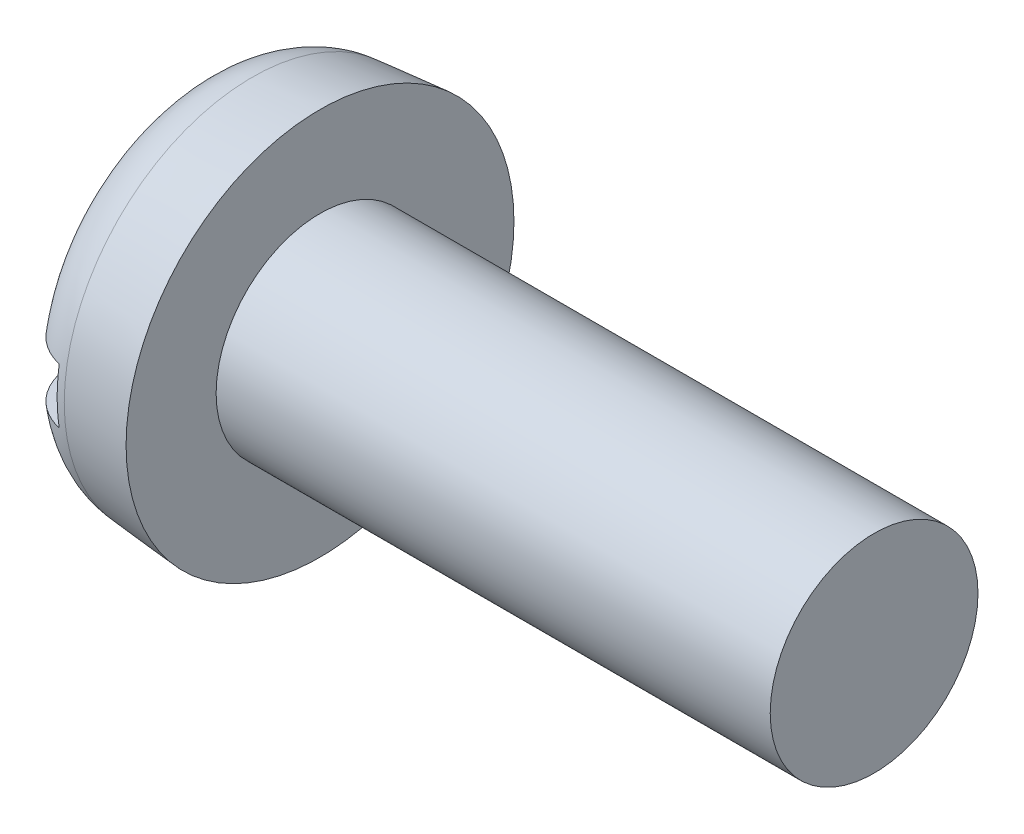
SolidWorks part; units mm, degrees
ref_plane "Plane1" through (0, 0, 0) normal (0, 0, 1) x (1, 0, 0)
ref_plane "Plane2" through (0, 0, 0) normal (0, 1, 0) x (1, 0, 0)
ref_plane "Plane3" through (0, 0, 0) normal (1, 0, 0) x (0, 0, -1)
sketch "BodySke" plane through (0, 0, 0) normal (0, 0, 1) x (1, 0, 0)
  line L0 (1.8, 1.5) -> (1.8, 2.8)
  line L1 (0, 0) -> (0, 2.6425)
  line L2 (-25.4, 0) -> (127, 0) construction
  line L3 (9.8, 0) -> (0, 0)
  line L4 (1.8, 1.5) -> (9.8, 1.5)
  line L5 (9.8, 1.5) -> (9.8, 0)
  line L6 (0, 2.6425) -> (1.8, 2.8)
  line L9 (2.3, 3.0875) -> (2.3, -6.4375) construction
  line L10 (1.8, 6.35) -> (1.8, -3.175) construction
revolve "Base-Revolve" add sketch "BodySke"
cosmetic thread "ThreadCosmetic" [suppressed]
fillet "Fillet1" [suppressed] radius 0.1
fillet "Fillet2" radius 0.9 1 edges at (0, 0, 2.6425)
sketch "Sketch2" plane through (0, 0, 0) normal (1, 0, 0) x (0, 0, -1)
  line L0 (2.8, -0.4) -> (-2.8, -0.4)
  line L1 (2.8, -0.4) -> (2.8, 0.4)
  line L2 (-2.8, 0.4) -> (2.8, 0.4)
  line L3 (-2.8, 0.4) -> (-2.8, -0.4)
extrude "Slot" cut sketch "Sketch2" along normal blind 0.7
sketch "ThdSchSke" plane through (0, 0, 0) normal (0, 0, 1) x (1, 0, 0)
  line L0 (2.8, -1.2195) -> (2.6036, -1.5)
  line L1 (2.8, -1.2195) -> (2.9964, -1.5)
  line L2 (2.9964, -1.5) -> (2.9964, -1.875)
  line L3 (-3.175, 0) -> (5.1513, 0) construction
  line L5 (2.9964, -1.875) -> (2.6036, -1.875)
  line L6 (2.6036, -1.875) -> (2.6036, -1.5)
revolve "ThreadSchematic" [suppressed] cut sketch "ThdSchSke" angle 360 about L3
pattern_linear "ThdSchPat" [suppressed]
equation "\"D1@Sketch2\" = \"Head_dia@BodySke\""
equation "\"D2@Sketch2\" = \"D1@Sketch2\" / 2"
equation "\"D3@Sketch2\" = \"Slot_width@Sketch2\" / 2"
equation "\"Thread_length@ThreadCosmetic\" = ((sgn( (\"Length@BodySke\" - \"Advance@BodySke\" * 2.0 ) - \"Thread_nom@BodySke\" )-1)*( (\"Length@BodySke\" - \"Advance@BodySke\"  * 2.0) - \"Thread_nom@BodySke\" ))/-2+ \"Thread_nom@BodySke\""
equation "\"Thread_minor@ThdSchSke\" = \"Thread_minor@ThreadCosmetic\""
equation "\"Diameter@ThdSchSke\" = \"Diameter@BodySke\""
equation "\"Overcut@ThdSchSke\" = \"Diameter@BodySke\" * 1.25"
equation "\"Start@ThdSchSke\" = \"Head_ht@BodySke\" + \"Length@BodySke\" - \"Thread_length@ThreadCosmetic\"  '---Non-countersunk---"
equation "\"Num_threads@ThdSchPat\" = int( \"Thread_length@ThreadCosmetic\" / \"Advance@BodySke\" + 0.999 )  + 1"
equation "\"Advance@ThdSchPat\" = \"Thread_length@ThreadCosmetic\" /  (\"Num_threads@ThdSchPat\" - 1) 'relax it"
